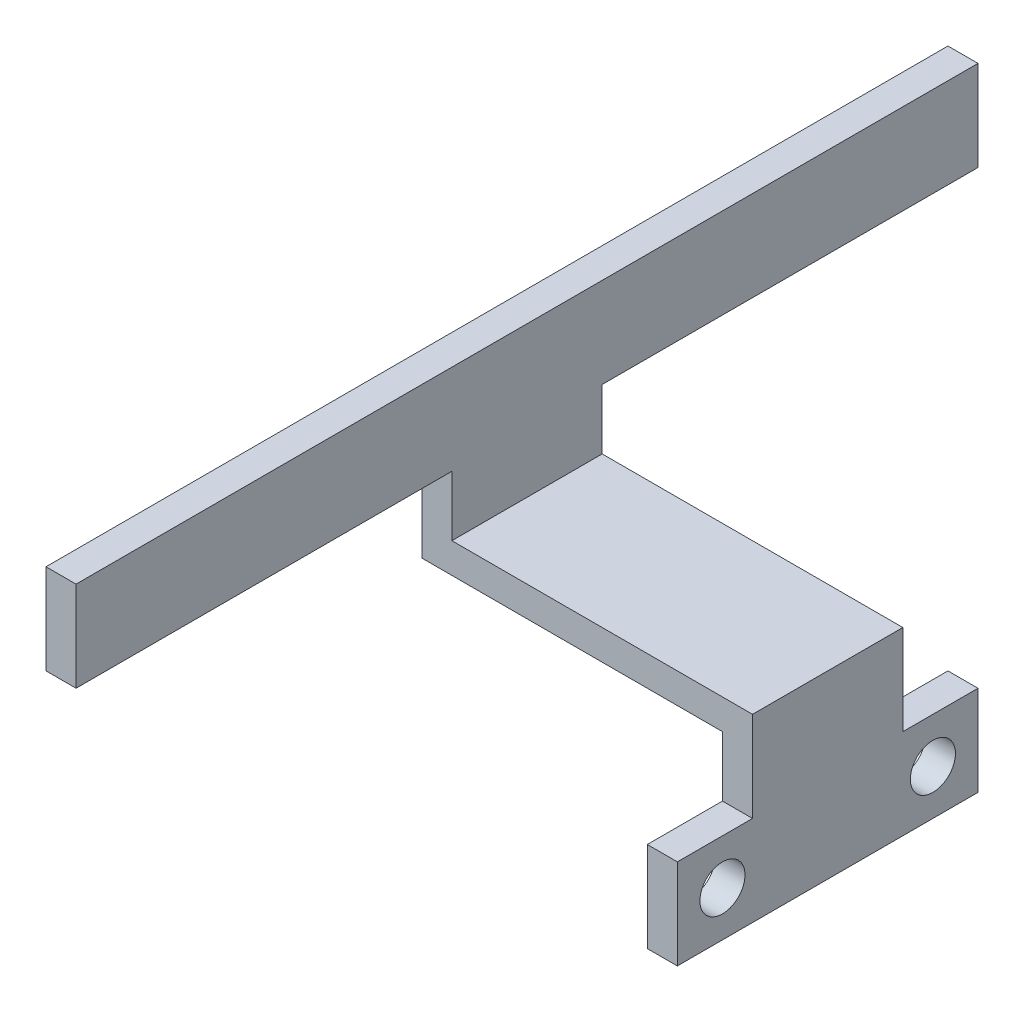
SolidWorks part; units mm, degrees
ref_plane "Front Plane" through (0, 0, 0) normal (0, 0, 1) x (1, 0, 0)
ref_plane "Top Plane" through (0, 0, 0) normal (0, 1, 0) x (1, 0, 0)
ref_plane "Right Plane" through (0, 0, 0) normal (1, 0, 0) x (0, 0, -1)
sketch "Sketch1" plane through (0, 0, 0) normal (0, 0, 1) x (1, 0, 0)
  line L0 (-14.2162, 5.6738) -> (-14.2162, 15.6738)
  line L1 (-16.2162, 3.6738) -> (3.7838, 3.6738)
  line L3 (-14.2162, 5.6738) -> (5.7838, 5.6738)
  line L8 (-16.2162, 3.6738) -> (-16.2162, 15.6738)
  line L9 (-16.2162, 15.6738) -> (-14.2162, 15.6738)
  line L10 (5.7838, 5.6738) -> (5.7838, -6.3262)
  line L11 (5.7838, -6.3262) -> (3.7838, -6.3262)
  line L12 (3.7838, -6.3262) -> (3.7838, 3.6738)
  point P0 (0, 0)
  dimension "D1" = 2
  dimension "D2" = 2
  dimension "D3" = 2
  dimension "D4" = 10
  dimension "D5" = 10
  dimension "D6" = 20
extrude "Boss-Extrude1" add sketch "Sketch1" along normal mid plane 10
sketch "Sketch2" plane through (5.7838, 0, 0) normal (1, 0, 0) x (0, 0, -1)
  line L0 (-10, -6.3262) -> (10, -6.3262)
  line L1 (10, -6.3262) -> (10, -0.3262)
  line L2 (10, -0.3262) -> (-10, -0.3262)
  line L3 (-10, -0.3262) -> (-10, -6.3262)
  circle A0 centre (-7, -3.3262) radius 1.5
  circle A1 centre (7, -3.3262) radius 1.5
  dimension "D3" = 3
  dimension "D4" = 3
  dimension "D5" = 3
  dimension "D6" = 3
  dimension "D7" = 3
  dimension "D8" = 3
  dimension "D1" = 20
  dimension "D2" = 10
  dimension "D9" = 6
extrude "Boss-Extrude2" add sketch "Sketch2" against normal blind 2
sketch "Sketch3" plane through (-16.2162, 0, 0) normal (-1, 0, 0) x (0, 0, 1)
  line L0 (-10, -0.3262) -> (-5, -0.3262) construction
  line L1 (-30, 15.6738) -> (30, 15.6738)
  line L2 (-30, 15.6738) -> (-30, 9.6738)
  line L3 (-30, 9.6738) -> (30, 9.6738)
  line L4 (30, 15.6738) -> (30, 9.6738)
  dimension "D1" = 60
  dimension "D2" = 30
  dimension "D3" = 6
  dimension "D4" = 10
extrude "Boss-Extrude3" add sketch "Sketch3" against normal blind 2
